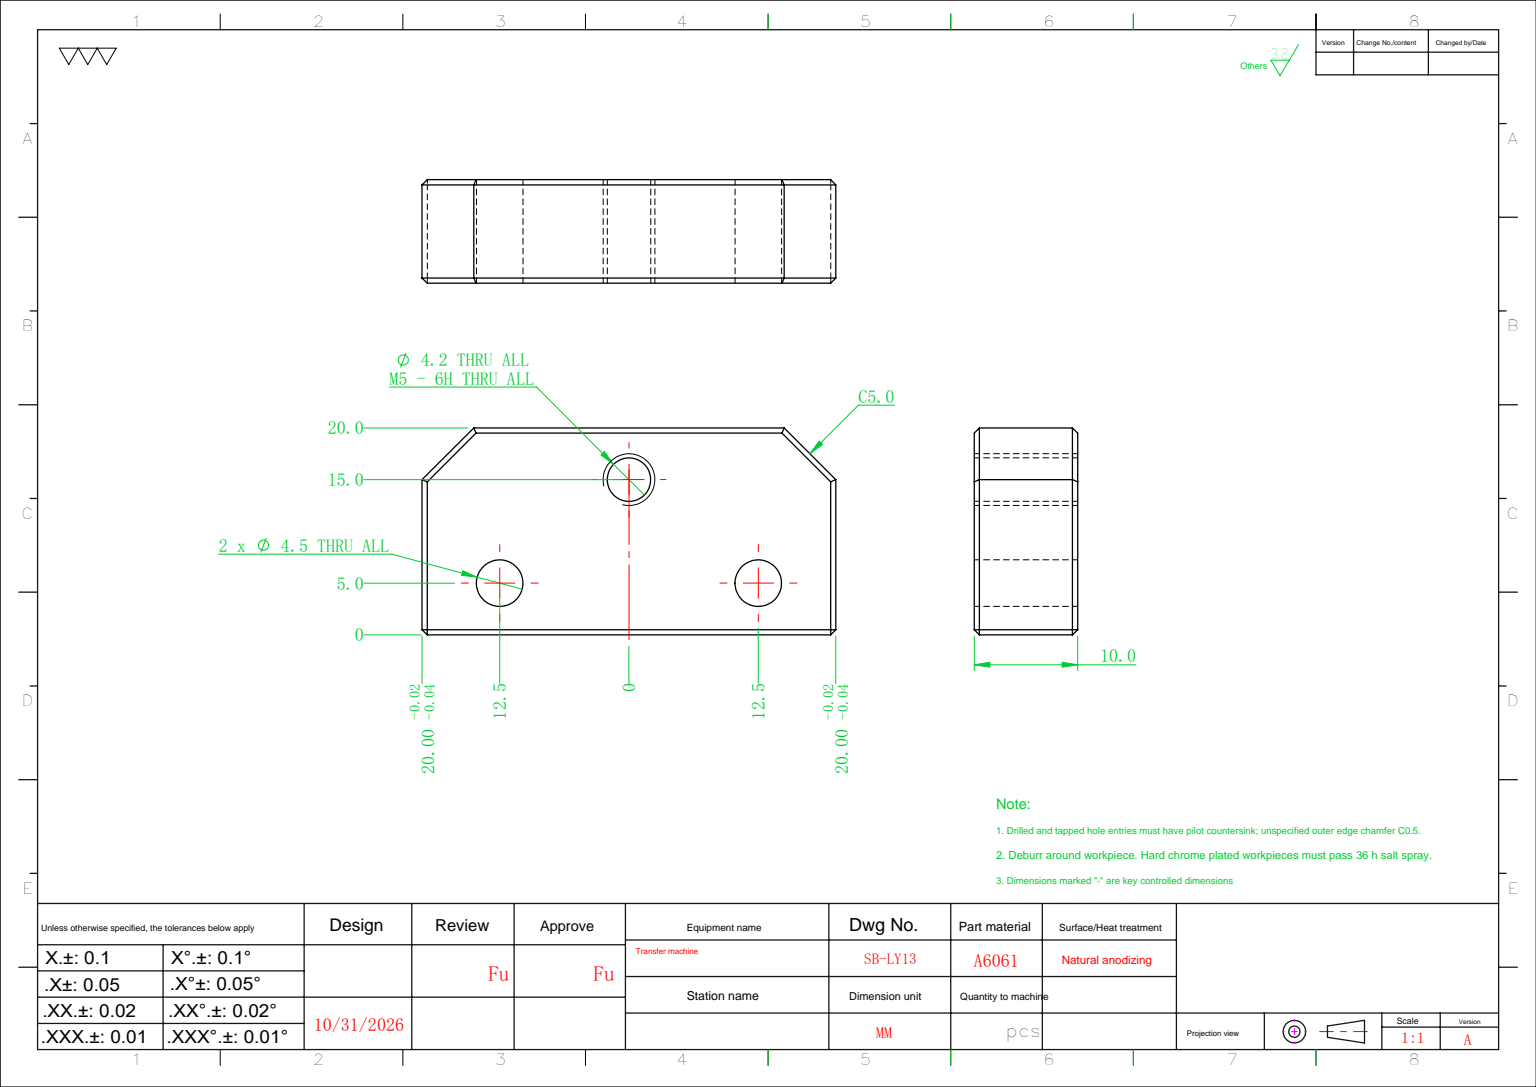
from build123d import *

# Parameters (mm, degrees)
SKETCH_1_W              = 40
SKETCH_1_H              = 20
EXTRUDE_1_DEPTH         = 10
HOLE_WIZARD_4_5_4_5_1_D = 4.5
HOLE_WIZARD_M5_1_D      = 4.2
CHAMFER_1_SIZE          = 5
CHAMFER_2_SIZE          = 0.5


with BuildPart() as part:
    # 草图1 → 凸台-拉伸1 (new body)
    with BuildSketch(Plane.XY):
        Rectangle(SKETCH_1_W, SKETCH_1_H)
    extrude(amount=EXTRUDE_1_DEPTH)

    # Ø4.5 (4.5) 直径孔1 (through all)
    with Locations(Plane.XY.offset(10)):
        with Locations((12.5, 5), (-12.5, 5)):
            Hole(HOLE_WIZARD_4_5_4_5_1_D / 2)

    # M5 螺纹孔1 (through all)
    with Locations(Plane.XY.offset(10)):
        with Locations((0, -5)):
            Hole(HOLE_WIZARD_M5_1_D / 2)

    # 倒角1
    chamfer_1_edges = [part.edges().sort_by_distance(p)[0] for p in [
        (20, -10, 5),
        (-20, -10, 5),
    ]]
    chamfer(chamfer_1_edges, length=CHAMFER_1_SIZE)

    # 倒角2
    chamfer_2_edges = [part.edges().sort_by_distance(p)[0] for p in [
        (-20, 2.5, 10),
        (0, -10, 0),
        (0, -10, 10),
        (20, 2.5, 0),
        (17.5, -7.5, 0),
        (-17.5, -7.5, 0),
        (20, 2.5, 10),
        (17.5, -7.5, 10),
        (-17.5, -7.5, 10),
        (-20, 2.5, 0),
        (0, 10, 0),
        (-20, 10, 5),
        (20, 10, 5),
        (0, 10, 10),
    ]]
    chamfer(chamfer_2_edges, length=CHAMFER_2_SIZE)


solid = part.part
